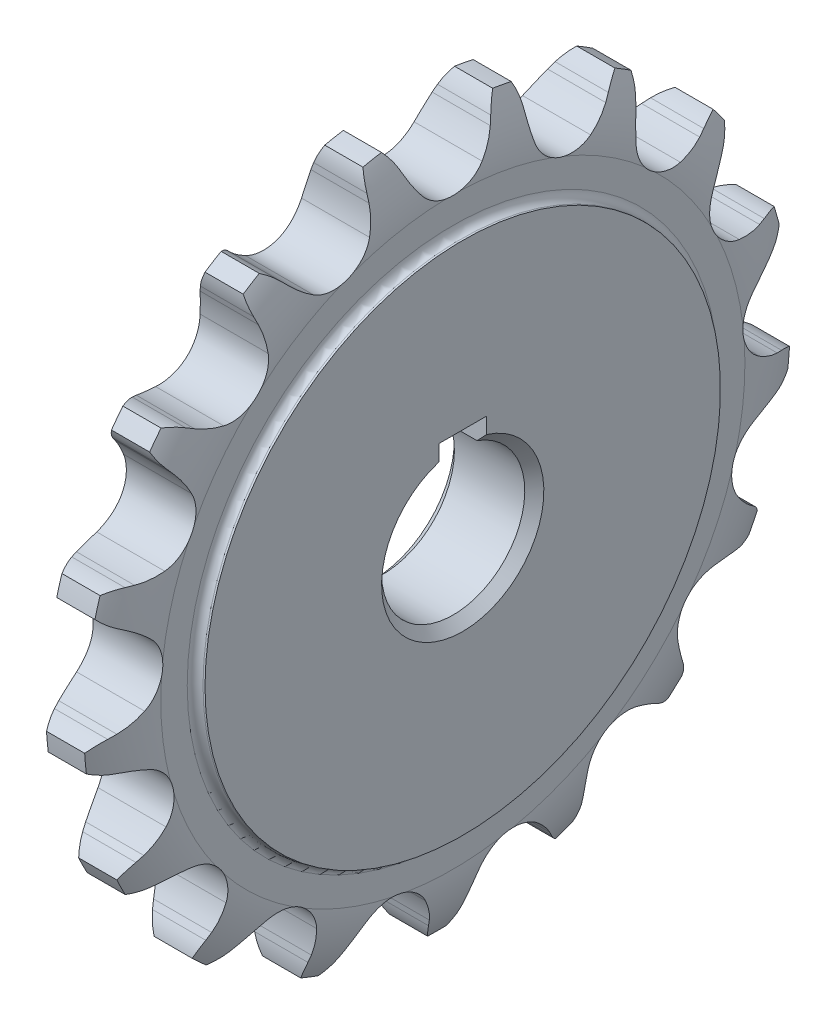
from build123d import *

# Parameters (mm, degrees)
CUT_EXTRUDE_1_DEPTH      = 4.685156443
PATTERN_CIRCULAR_1_COUNT = 17
SKETCH_4_W               = 5
SKETCH_4_H               = 2.72893214
CUT_EXTRUDE_2_DEPTH      = 54.102851886
CHAMFER_1_SIZE           = 1
CHAMFER_2_SIZE           = 1


with BuildPart() as part:
    # 草图1 → 旋转1 (revolve)
    with BuildSketch(Plane.XY, mode=Mode.PRIVATE) as revolve_1_sk:
        with BuildLine():
            Line((-4.685156443, 7.5), (-4.685156443, 27))
            Line((-4.685156443, 27), (-4.478175154, 27))
            ThreePointArc((-4.478175154, 27), (-3.892743663, 27.242493663), (-3.65025, 27.827925154))
            Line((-3.65025, 27.827925154), (-3.65025, 30.597913814))
            ThreePointArc((-3.65025, 30.597913814), (-3.248667458, 33.908278728), (-1.99925, 37))
            Line((-1.99925, 37), (1.99925, 37))
            ThreePointArc((1.99925, 37), (3.248667458, 33.908278728), (3.65025, 30.597913814))
            Line((3.65025, 30.597913814), (3.65025, 27.827925154))
            ThreePointArc((3.65025, 27.827925154), (3.892743663, 27.242493663), (4.478175154, 27))
            Line((4.478175154, 27), (4.685156443, 27))
            Line((4.685156443, 27), (4.685156443, 7.5))
            Line((4.685156443, 7.5), (-4.685156443, 7.5))
        make_face()
    revolve(revolve_1_sk.sketch.rotate(Axis((-6.35, 0, 0), (1, 0, 0)), 90), axis=Axis((-6.35, 0, 0), (1, 0, 0)))

    # 草图2 → 切除-拉伸1 (cut, symmetric)
    with BuildSketch(Plane(origin=(0, 0, 0), x_dir=(0, 0, -1), z_dir=(1, 0, 0))):
        with BuildLine():
            Line((4.525990365, 34.317747091), (4.828460685, 35.00277706))
            ThreePointArc((4.828460685, 35.00277706), (5.264672951, 35.810417906), (5.823136285, 36.538898229))
            ThreePointArc((5.823136285, 36.538898229), (0, 37), (-5.823136285, 36.538898229))
            ThreePointArc((-5.823136285, 36.538898229), (-5.264672951, 35.810417906), (-4.828460685, 35.00277706))
            Line((-4.828460685, 35.00277706), (-4.525990365, 34.317747091))
            ThreePointArc((-4.525990365, 34.317747091), (-3.912159361, 33.138588704), (-3.152466185, 32.047685738))
            ThreePointArc((-3.152466185, 32.047685738), (0, 30.528113814), (3.152466185, 32.047685738))
            ThreePointArc((3.152466185, 32.047685738), (3.912159361, 33.138588704), (4.525990365, 34.317747091))
        make_face()
    cut_extrude_1 = extrude(amount=CUT_EXTRUDE_1_DEPTH, both=True, mode=Mode.SUBTRACT)

    # 阵列(圆周)1: 切除-拉伸1 ×17 about axis
    pattern_circular_1_axis = Axis((0, 0, 0), (1, 0, 0))
    for i in range(1, PATTERN_CIRCULAR_1_COUNT):
        add(cut_extrude_1.rotate(pattern_circular_1_axis, i * 360 / PATTERN_CIRCULAR_1_COUNT), mode=Mode.SUBTRACT)

    # 草图4 → 切除-拉伸2 (cut, through all)
    with BuildSketch(Plane.ZY.offset(4.685156443)):
        with Locations((0, 8.435533882)):
            Rectangle(SKETCH_4_W, SKETCH_4_H)
    extrude(amount=-CUT_EXTRUDE_2_DEPTH, mode=Mode.SUBTRACT)

    # 倒角1
    chamfer_1_edges = [part.edges().sort_by_distance(p)[0] for p in [
        (-4.685156443, -7.5, 0),
    ]]
    chamfer(chamfer_1_edges, length=CHAMFER_1_SIZE)

    # 倒角2
    chamfer_2_edges = [part.edges().sort_by_distance(p)[0] for p in [
        (4.685156443, -7.5, 0),
    ]]
    chamfer(chamfer_2_edges, length=CHAMFER_2_SIZE)


solid = part.part
